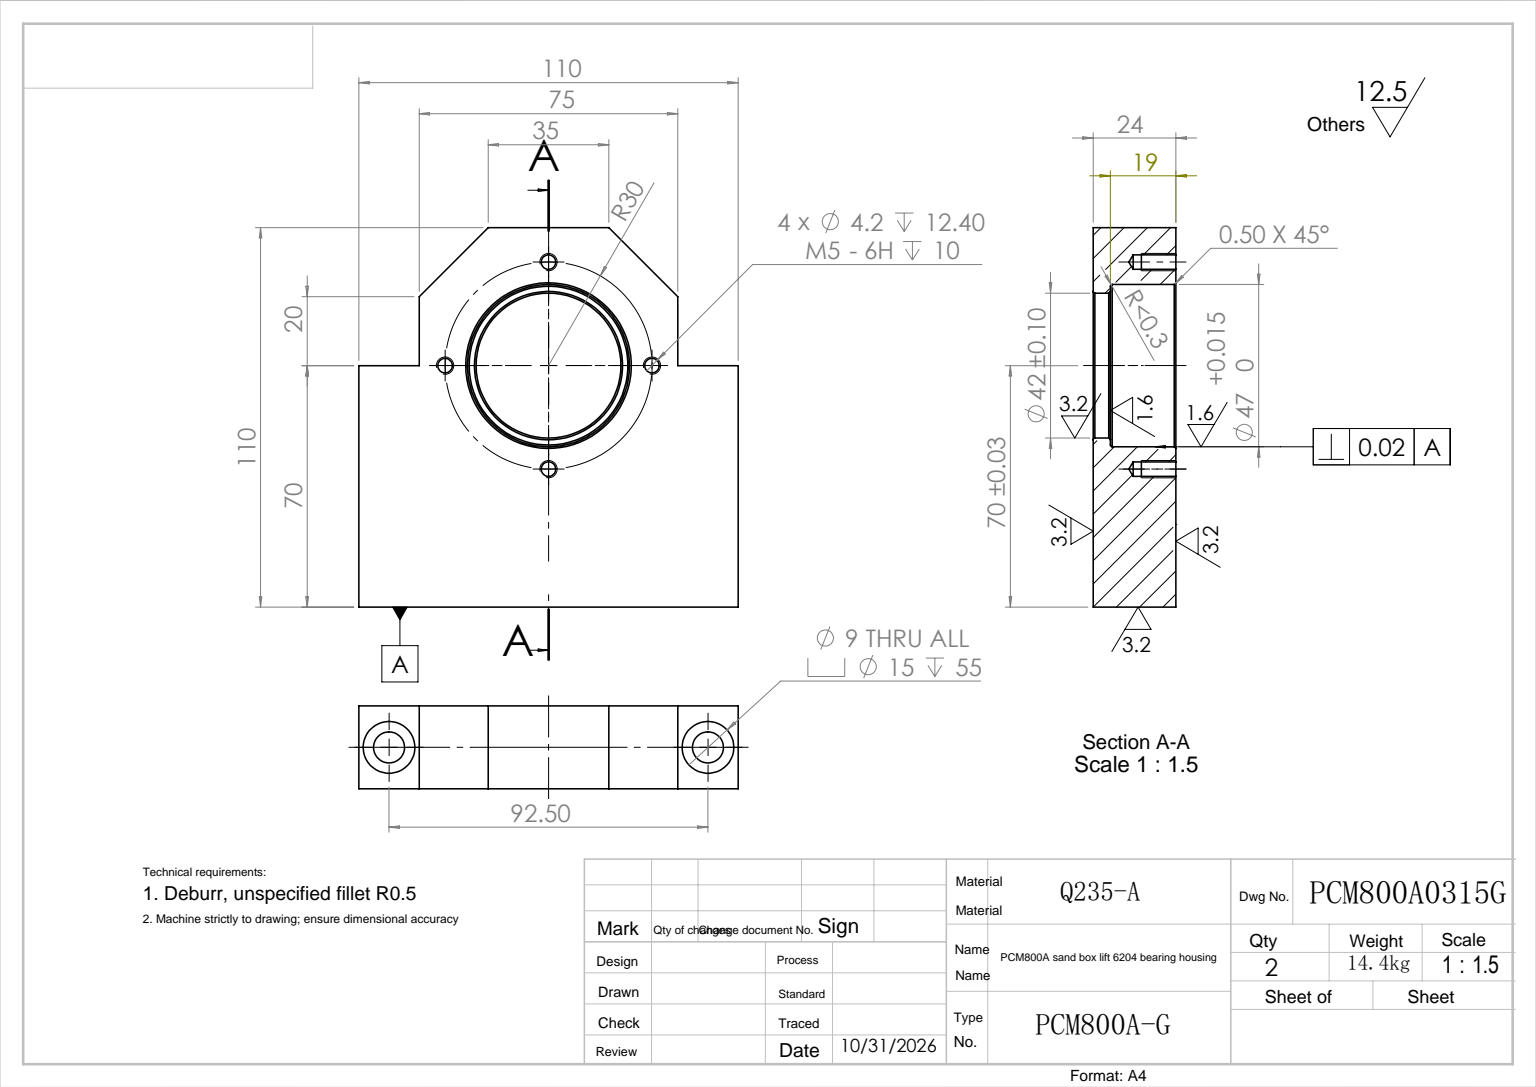
from build123d import *

# Parameters (mm, degrees)
SKETCH_1_W                = 110
SKETCH_1_H                = 24
EXTRUDE_1_DEPTH           = 110
SKETCH_2_R                = 21
CUT_EXTRUDE_1_DEPTH       = 5
SKETCH_3_R                = 23.5
CUT_EXTRUDE_2_DEPTH       = 19
SKETCH_5_W                = 17.5
SKETCH_5_H                = 40
CUT_EXTRUDE_3_DEPTH       = 158.40393896
CHAMFER_1_SIZE            = 20
HOLE_WIZARD_M5_1_D        = 4.2
HOLE_WIZARD_M5_1_DEPTH    = 12.4
HOLE_WIZARD_M5_1_TIP      = 1.2618073
HOLE_WIZARD_1_D           = 9
HOLE_WIZARD_1_CBORE_D     = 15
HOLE_WIZARD_1_CBORE_DEPTH = 55
FILLET_2_R                = 0.5
CHAMFER_2_SIZE            = 0.5


with BuildPart() as part:
    # 草图1 → 拉伸1 (new body)
    with BuildSketch(Plane(origin=(0, 0, 0), x_dir=(1, 0, 0), z_dir=(0, 1, 0))):
        with Locations((55, 12)):
            Rectangle(SKETCH_1_W, SKETCH_1_H)
    extrude(amount=EXTRUDE_1_DEPTH)

    # 草图2 → 切除-拉伸1 (cut)
    with BuildSketch(Plane.XY):
        with Locations((55, 70)):
            Circle(SKETCH_2_R)
    extrude(amount=-CUT_EXTRUDE_1_DEPTH, mode=Mode.SUBTRACT)

    # 草图3 → 切除-拉伸2 (cut)
    with BuildSketch(Plane.XY.offset(-5)):
        with Locations((55, 70)):
            Circle(SKETCH_3_R)
    extrude(amount=-CUT_EXTRUDE_2_DEPTH, mode=Mode.SUBTRACT)

    # 草图5 → 切除-拉伸3 (cut, through all)
    with BuildSketch(Plane(origin=(0, 0, -24), x_dir=(-1, 0, 0), z_dir=(0, 0, -1))):
        with Locations((-101.25, 90)):
            Rectangle(SKETCH_5_W, SKETCH_5_H)
        with Locations((-8.75, 90)):
            Rectangle(SKETCH_5_W, SKETCH_5_H)
    extrude(amount=-CUT_EXTRUDE_3_DEPTH, mode=Mode.SUBTRACT)

    # 倒角1
    chamfer_1_edges = [part.edges().sort_by_distance(p)[0] for p in [
        (92.5, 110, -12),
        (17.5, 110, -12),
    ]]
    chamfer(chamfer_1_edges, length=CHAMFER_1_SIZE)

    # M5 螺纹孔1
    with Locations(Plane(origin=(55, 100, -24), x_dir=(-1, 0, 0), z_dir=(0, 0, -1))):
        with Locations((0, 0), (-30, -30), (0, -60), (30, -30)):
            Hole(HOLE_WIZARD_M5_1_D / 2, depth=HOLE_WIZARD_M5_1_DEPTH)
            with Locations((0, 0, -(HOLE_WIZARD_M5_1_DEPTH + HOLE_WIZARD_M5_1_TIP / 2))):  # 118° drill point
                Cone(0, HOLE_WIZARD_M5_1_D / 2, HOLE_WIZARD_M5_1_TIP, mode=Mode.SUBTRACT)

    # 打孔尺寸根据内六角圆柱头螺钉的类型1 (through all)
    with Locations(Plane(origin=(8.75, 70, -12), x_dir=(0, 0, 1), z_dir=(0, 1, 0))):
        with Locations((0, 0), (0, 92.5)):
            CounterBoreHole(HOLE_WIZARD_1_D / 2, HOLE_WIZARD_1_CBORE_D / 2, HOLE_WIZARD_1_CBORE_DEPTH)

    # 圆角2
    fillet_2_edges = [part.edges().sort_by_distance(p)[0] for p in [
        (34, 70, 0),
        (31.5, 70, -5),
        (34, 70, -5),
    ]]
    fillet(fillet_2_edges, radius=FILLET_2_R)

    # 倒角2
    chamfer_2_edges = [part.edges().sort_by_distance(p)[0] for p in [
        (31.5, 70, -24),
    ]]
    chamfer(chamfer_2_edges, length=CHAMFER_2_SIZE)


solid = part.part
